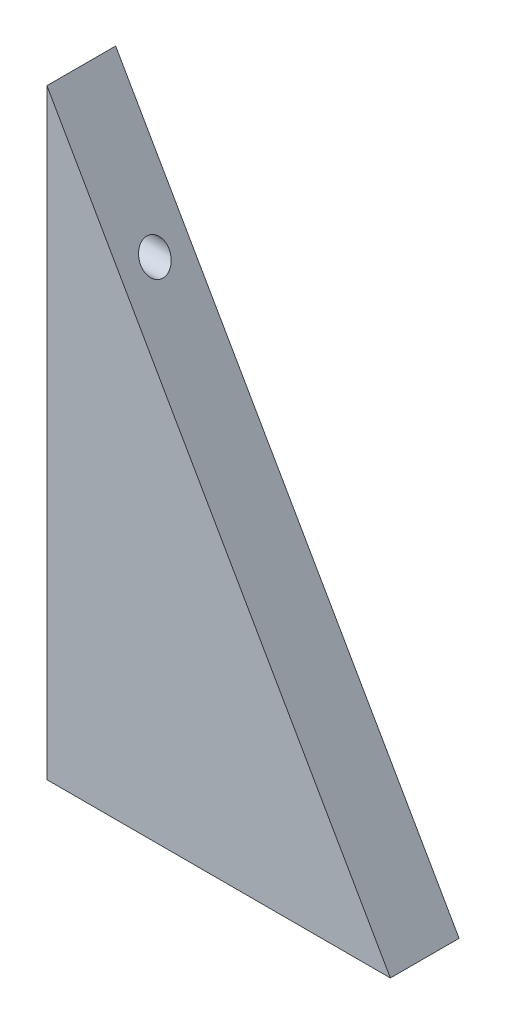
SolidWorks part; units mm, degrees
ref_plane "前视基准面" through (0, 0, 0) normal (0, 0, 1) x (1, 0, 0)
ref_plane "上视基准面" through (0, 0, 0) normal (0, 1, 0) x (1, 0, 0)
ref_plane "右视基准面" through (0, 0, 0) normal (1, 0, 0) x (0, 0, -1)
sketch "草图1" plane through (0, 0, 0) normal (0, 0, 1) x (1, 0, 0)
  line L0 (-20, -35) -> (20, -35)
  line L1 (20, -35) -> (-20, 35)
  line L2 (-20, 35) -> (-20, -35)
  dimension "D1" = 70
  dimension "D2" = 40
  dimension "D3" = 35
  dimension "D4" = 20
extrude "凸台-拉伸1" add sketch "草图1" along normal blind 8
hole_wizard "M4 螺纹孔1" positions "草图2" profile "草图3" tap size "M4" standard "ISO"
sketch "草图2" plane through (-20, 0, 0) normal (-1, 0, 0) x (0, 0, 1)
  line L0 (4, -35) -> (4, 35) construction
  line L1 (8, -35) -> (0, -35) construction
  line L2 (8, 35) -> (0, 35) construction
  line L3 (0, 0) -> (8, 0) construction
  line L4 (8, 35) -> (8, -35) construction
  point P0 (4, -20)
  point P2 (4, 0)
  point P4 (4, 20)
  dimension "D1" = 20
  dimension "D2" = 20
cosmetic thread "孔螺蚊线1"
cosmetic thread "孔螺蚊线2"
cosmetic thread "孔螺蚊线3"
sketch "草图3" plane through (-20, -20, 4) normal (0, 1, 0) x (0, 0, 1)
  line L0 (0, 0) -> (0, 12.9914)
  line L1 (0, 12.9914) -> (1.65, 12)
  line L2 (1.65, 12) -> (1.65, 0)
  line L5 (1.65, 0) -> (0, 0)
  line L10 (0, 12.9914) -> (-1.65, 12) construction
  line L11 (0, -6.35) -> (0, 107.95) construction
  dimension "螺纹孔钻头直径" = 3.3
  dimension "螺纹孔钻头深度" = 12
  dimension "导头角度" = 118
hole_wizard "M4 螺纹孔2" positions "草图4" profile "草图5" tap size "M4" standard "ISO"
sketch "草图4" plane through (0, -35, 0) normal (0, -1, 0) x (-1, 0, 0)
  line L0 (-20, -4) -> (20, -4) construction
  line L1 (-20, -8) -> (-20, 0) construction
  line L2 (20, -8) -> (20, 0) construction
  line L4 (0, 0) -> (0, -8) construction
  line L5 (20, 0) -> (-20, 0) construction
  line L6 (20, -8) -> (-20, -8) construction
  point P0 (-10, -4)
  point P2 (10, -4)
  dimension "D1" = 20
sketch "草图5" plane through (10, -35, 4) normal (1, 0, 0) x (0, 0, -1)
  line L0 (0, 0) -> (0, 12.9914)
  line L1 (0, 12.9914) -> (1.65, 12)
  line L2 (1.65, 12) -> (1.65, 0)
  line L5 (1.65, 0) -> (0, 0)
  line L10 (0, 12.9914) -> (-1.65, 12) construction
  line L11 (0, -6.35) -> (0, 107.95) construction
  dimension "螺纹孔钻头直径" = 3.3
  dimension "螺纹孔钻头深度" = 12
  dimension "导头角度" = 118
cosmetic thread "孔螺蚊线4"
cosmetic thread "孔螺蚊线5"
